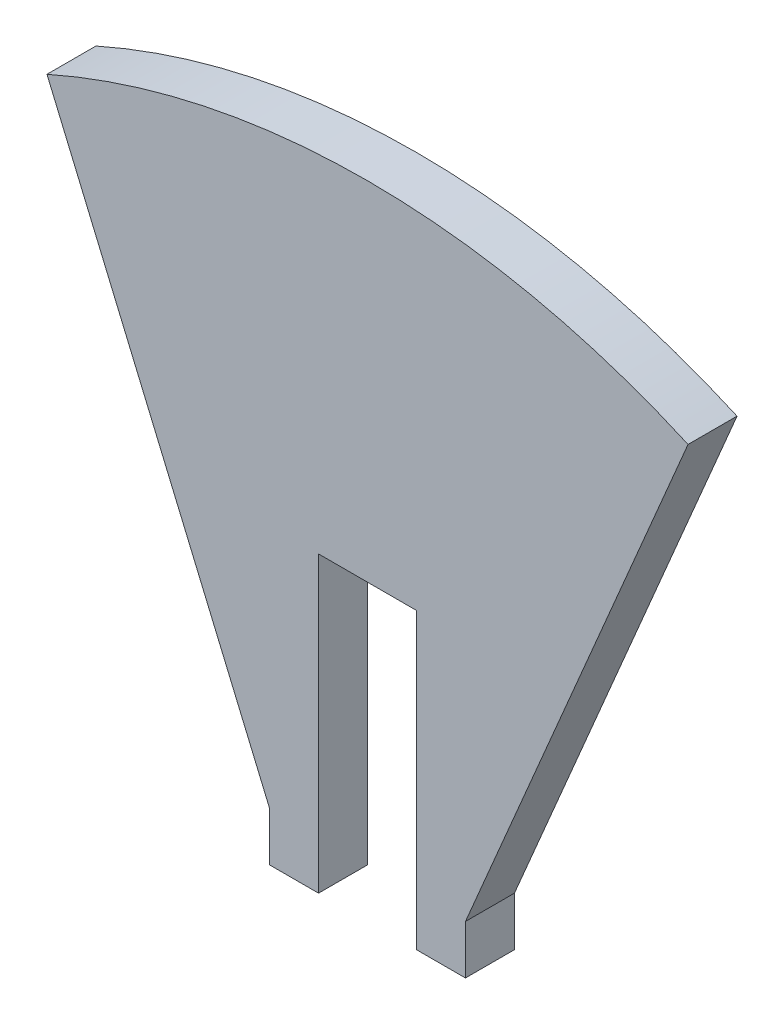
SolidWorks part; units mm, degrees
ref_plane "Front Plane" through (0, 0, 0) normal (0, 0, 1) x (1, 0, 0)
ref_plane "Top Plane" through (0, 0, 0) normal (0, 1, 0) x (1, 0, 0)
ref_plane "Right Plane" through (0, 0, 0) normal (1, 0, 0) x (0, 0, -1)
sketch "Sketch1" plane through (0, 0, 0) normal (0, 0, 1) x (1, 0, 0)
  line L0 (0, 161) -> (0, -161) construction
  line L1 (-65.4581, 147.0926) -> (-20, 40)
  line L2 (-20, 40) -> (-20, 30)
  line L3 (-20, 30) -> (20, 30)
  line L4 (20, 30) -> (20, 40)
  line L5 (20, 40) -> (65.4581, 147.0926)
  arc A0 (65.4581, 147.0926) -> (-65.4581, 147.0926) centre (0, 0) ccw
  dimension "D3" = 322
  dimension "D1" = 46
  dimension "D2" = 30
  dimension "D4" = 10
  dimension "D5" = 40
extrude "Boss-Extrude1" add sketch "Sketch1" along normal mid plane 10
sketch "Sketch2" plane through (0, 0, 5) normal (0, 0, 1) x (1, 0, 0)
  line L0 (-20, 30) -> (20, 30) construction
  line L1 (10, -30) -> (-10, -30)
  line L2 (10, -30) -> (10, 90)
  line L3 (10, 90) -> (-10, 90)
  line L4 (-10, -30) -> (-10, 90)
  line L5 (10, -30) -> (-10, 90) construction
  line L6 (10, 90) -> (-10, -30) construction
  point P0 (0, 30)
  dimension "D1" = 20
  dimension "D2" = 60
extrude "Cut-Extrude1" cut sketch "Sketch2" against normal blind 10
